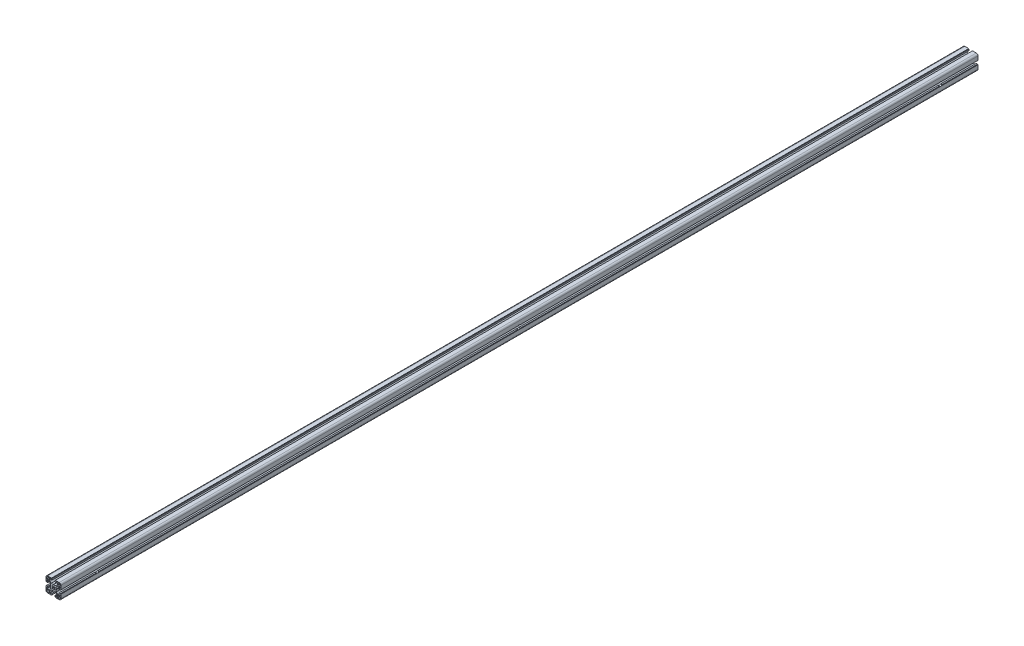
SolidWorks part; units mm, degrees
material "6061 GB/T6892-2006"
ref_plane "前视" through (0, 0, 0) normal (0, 0, 1) x (1, 0, 0)
ref_plane "上视" through (0, 0, 0) normal (0, 1, 0) x (1, 0, 0)
ref_plane "右视" through (0, 0, 0) normal (1, 0, 0) x (0, 0, -1)
sketch "草图1" plane through (0, 0, 0) normal (0, 0, 1) x (1, 0, 0)
  line L0 (-18.9995, -4.1003) -> (-18.9995, -5.1003)
  line L1 (-18.9995, -5.1003) -> (-19.9995, -5.1003)
  line L2 (-19.9995, -5.1003) -> (-19.9995, -15.5003)
  line L3 (-15.4995, -20.0003) -> (-5.0995, -20.0003)
  line L4 (-5.0995, -20.0003) -> (-5.0995, -19.0003)
  line L5 (-5.0995, -19.0003) -> (-4.0995, -19.0003)
  line L6 (-4.0995, -19.0003) -> (-4.0995, -15.5003)
  line L7 (-4.0995, -15.5003) -> (-6.5995, -15.5003)
  line L8 (-6.5995, -15.5003) -> (-6.5995, -16.5003)
  line L9 (-7.5995, -17.5003) -> (-9.7995, -17.5003)
  line L10 (-10.2995, -17.0003) -> (-10.2995, -11.9973)
  line L11 (-10.2995, -11.9973) -> (-5.9025, -7.6003)
  line L12 (-5.9025, -7.6003) -> (-0.5195, -7.6003)
  line L13 (-0.5195, -7.6003) -> (0.0005, -7.3003)
  line L14 (0.0005, -7.3003) -> (0.5195, -7.6003)
  line L15 (0.5195, -7.6003) -> (5.9035, -7.6003)
  line L16 (5.9035, -7.6003) -> (10.3005, -11.9973)
  line L17 (10.3005, -11.9973) -> (10.3005, -17.0003)
  line L18 (9.8005, -17.5003) -> (7.6005, -17.5003)
  line L19 (6.6005, -16.5003) -> (6.6005, -15.5003)
  line L20 (6.6005, -15.5003) -> (4.1005, -15.5003)
  line L21 (4.1005, -15.5003) -> (4.1005, -19.0003)
  line L22 (4.1005, -19.0003) -> (5.1005, -19.0003)
  line L23 (5.1005, -19.0003) -> (5.1005, -20.0003)
  line L24 (5.1005, -20.0003) -> (15.5005, -20.0003)
  line L25 (20.0005, -15.5003) -> (20.0005, -5.1003)
  line L26 (20.0005, -5.1003) -> (19.0005, -5.1003)
  line L27 (19.0005, -5.1003) -> (19.0005, -4.1003)
  line L28 (19.0005, -4.1003) -> (15.5005, -4.1003)
  line L29 (15.5005, -4.1003) -> (15.5005, -6.6003)
  line L30 (15.5005, -6.6003) -> (16.5005, -6.6003)
  line L31 (17.5005, -7.6003) -> (17.5005, -9.8003)
  line L32 (17.0005, -10.3003) -> (11.9975, -10.3003)
  line L33 (11.9975, -10.3003) -> (7.6005, -5.9033)
  line L34 (7.6005, -5.9033) -> (7.6005, -0.5203)
  line L35 (7.6005, -0.5203) -> (7.3005, -0.0003)
  line L36 (7.3005, -0.0003) -> (7.6005, 0.5197)
  line L37 (7.6005, 0.5197) -> (7.6005, 5.9027)
  line L38 (7.6005, 5.9027) -> (11.9975, 10.2997)
  line L39 (11.9975, 10.2997) -> (17.0005, 10.2997)
  line L40 (17.5005, 9.7997) -> (17.5005, 7.5997)
  line L41 (16.5005, 6.5997) -> (15.5005, 6.5997)
  line L42 (15.5005, 6.5997) -> (15.5005, 4.0997)
  line L43 (15.5005, 4.0997) -> (19.0005, 4.0997)
  line L44 (19.0005, 4.0997) -> (19.0005, 5.0997)
  line L45 (19.0005, 5.0997) -> (20.0005, 5.0997)
  line L46 (20.0005, 5.0997) -> (20.0005, 15.4997)
  line L47 (15.5005, 19.9997) -> (5.1005, 19.9997)
  line L48 (5.1005, 19.9997) -> (5.1005, 18.9997)
  line L49 (5.1005, 18.9997) -> (4.1005, 18.9997)
  line L50 (4.1005, 18.9997) -> (4.1005, 15.4997)
  line L51 (4.1005, 15.4997) -> (6.6005, 15.4997)
  line L52 (7.6005, 17.4997) -> (9.8005, 17.4997)
  line L53 (10.3005, 16.9997) -> (10.3005, 11.9967)
  line L54 (10.3005, 11.9967) -> (5.9035, 7.5997)
  line L55 (5.9035, 7.5997) -> (0.5195, 7.5997)
  line L56 (0.5195, 7.5997) -> (0.0005, 7.2997)
  line L57 (0.0005, 7.2997) -> (-0.5195, 7.5997)
  line L58 (-0.5195, 7.5997) -> (-5.9025, 7.5997)
  line L59 (-5.9025, 7.5997) -> (-10.2995, 11.9967)
  line L60 (-10.2995, 11.9967) -> (-10.2995, 16.9997)
  line L61 (-9.7995, 17.4997) -> (-7.5995, 17.4997)
  line L62 (-6.5995, 16.4997) -> (-6.5995, 15.4997)
  line L63 (-6.5995, 15.4997) -> (-4.0995, 15.4997)
  line L64 (-4.0995, 15.4997) -> (-4.0995, 18.9997)
  line L65 (-4.0995, 18.9997) -> (-5.0995, 18.9997)
  line L66 (-5.0995, 18.9997) -> (-5.0995, 19.9997)
  line L67 (-5.0995, 19.9997) -> (-15.4995, 19.9997)
  line L68 (-19.9995, 15.4997) -> (-19.9995, 5.0997)
  line L69 (-19.9995, 5.0997) -> (-18.9995, 5.0997)
  line L70 (-18.9995, 5.0997) -> (-18.9995, 4.0997)
  line L71 (-18.9995, 4.0997) -> (-15.4995, 4.0997)
  line L72 (-15.4995, 4.0997) -> (-15.4995, 6.5997)
  line L73 (-15.4995, 6.5997) -> (-16.4995, 6.5997)
  line L74 (-17.4995, 7.5997) -> (-17.4995, 9.7997)
  line L75 (-16.9995, 10.2997) -> (-11.9965, 10.2997)
  line L76 (-11.9965, 10.2997) -> (-7.5995, 5.9027)
  line L77 (-7.5995, 5.9027) -> (-7.5995, 0.5197)
  line L78 (-7.5995, 0.5197) -> (-7.2995, -0.0003)
  line L79 (-7.2995, -0.0003) -> (-7.5995, -0.5203)
  line L80 (-7.5995, -0.5203) -> (-7.5995, -5.9033)
  line L81 (-7.5995, -5.9033) -> (-11.9965, -10.3003)
  line L82 (-11.9965, -10.3003) -> (-16.9995, -10.3003)
  line L83 (-17.4995, -9.8003) -> (-17.4995, -7.6003)
  line L84 (-16.4995, -6.6003) -> (-15.4995, -6.6003)
  line L85 (-15.4995, -6.6003) -> (-15.4995, -4.1003)
  line L86 (-15.4995, -4.1003) -> (-18.9995, -4.1003)
  line L87 (15.5005, -18.0003) -> (11.8005, -18.0003)
  line L88 (11.8005, -18.0003) -> (11.8005, -11.8003)
  line L89 (11.8005, -11.8003) -> (18.0005, -11.8003)
  line L90 (18.0005, -11.8003) -> (18.0005, -15.5003)
  line L91 (18.0005, 11.7997) -> (11.8005, 11.7997)
  line L92 (11.8005, 11.7997) -> (11.8005, 17.9997)
  line L93 (11.8005, 17.9997) -> (15.5005, 17.9997)
  line L94 (18.0005, 15.4997) -> (18.0005, 11.7997)
  line L95 (-1.8145, -2.8753) -> (-3.0044, -4.0665)
  line L96 (-3.0044, -4.0665) -> (-4.0656, -3.0052)
  line L97 (-4.0656, -3.0052) -> (-2.8745, -1.8153)
  line L98 (-2.8745, 1.8147) -> (-4.0644, 3.0058)
  line L99 (-4.0644, 3.0058) -> (-3.0044, 4.0658)
  line L100 (-3.0044, 4.0658) -> (-1.8145, 2.8747)
  line L101 (1.8145, 2.8747) -> (3.0055, 4.0657)
  line L102 (3.0055, 4.0657) -> (4.0666, 3.0045)
  line L103 (4.0666, 3.0045) -> (2.8755, 1.8147)
  line L104 (2.8755, -1.8153) -> (4.0666, -3.0052)
  line L105 (4.0666, -3.0052) -> (3.0055, -4.0663)
  line L106 (3.0055, -4.0663) -> (1.8145, -2.8753)
  line L107 (-17.9995, -15.5003) -> (-17.9995, -11.8003)
  line L108 (-17.9995, -11.8003) -> (-11.7995, -11.8003)
  line L109 (-11.7995, -11.8003) -> (-11.7995, -18.0003)
  line L110 (-11.7995, -18.0003) -> (-15.4995, -18.0003)
  line L111 (-11.7995, 17.9997) -> (-11.7995, 11.7997)
  line L112 (-11.7995, 11.7997) -> (-17.9995, 11.7997)
  line L113 (-17.9995, 11.7997) -> (-17.9995, 15.4997)
  line L114 (-15.4995, 17.9997) -> (-11.7995, 17.9997)
  arc A0 (-19.9995, -15.5003) -> (-15.4995, -20.0003) centre (-15.4995, -15.5003) ccw
  arc A1 (-6.5995, -16.5003) -> (-7.5995, -17.5003) centre (-7.5995, -16.5003) cw
  arc A2 (-9.7995, -17.5003) -> (-10.2995, -17.0003) centre (-9.7995, -17.0003) cw
  arc A3 (10.3005, -17.0003) -> (9.8005, -17.5003) centre (9.8005, -17.0003) cw
  arc A4 (7.6005, -17.5003) -> (6.6005, -16.5003) centre (7.6005, -16.5003) cw
  arc A5 (15.5005, -20.0003) -> (20.0005, -15.5003) centre (15.5005, -15.5003) ccw
  arc A6 (16.5005, -6.6003) -> (17.5005, -7.6003) centre (16.5005, -7.6003) cw
  arc A7 (17.5005, -9.8003) -> (17.0005, -10.3003) centre (17.0005, -9.8003) cw
  arc A8 (17.0005, 10.2997) -> (17.5005, 9.7997) centre (17.0005, 9.7997) cw
  arc A9 (17.5005, 7.5997) -> (16.5005, 6.5997) centre (16.5005, 7.5997) cw
  arc A10 (20.0005, 15.4997) -> (15.5005, 19.9997) centre (15.5005, 15.4997) ccw
  arc A11 (6.6005, 15.4997) -> (6.6005, 16.4997) centre (7.1003, 15.9997) cw
  arc A12 (6.6005, 16.4997) -> (7.6005, 17.4997) centre (7.6005, 16.4997) cw
  arc A13 (9.8005, 17.4997) -> (10.3005, 16.9997) centre (9.8005, 16.9997) cw
  arc A14 (-10.2995, 16.9997) -> (-9.7995, 17.4997) centre (-9.7995, 16.9997) cw
  arc A15 (-7.5995, 17.4997) -> (-6.5995, 16.4997) centre (-7.5995, 16.4997) cw
  arc A16 (-15.4995, 19.9997) -> (-19.9995, 15.4997) centre (-15.4995, 15.4997) ccw
  arc A17 (-16.4995, 6.5997) -> (-17.4995, 7.5997) centre (-16.4995, 7.5997) cw
  arc A18 (-17.4995, 9.7997) -> (-16.9995, 10.2997) centre (-16.9995, 9.7997) cw
  arc A19 (-16.9995, -10.3003) -> (-17.4995, -9.8003) centre (-16.9995, -9.8003) cw
  arc A20 (-17.4995, -7.6003) -> (-16.4995, -6.6003) centre (-16.4995, -7.6003) cw
  arc A21 (18.0005, -15.5003) -> (15.5005, -18.0003) centre (15.5005, -15.5003) cw
  arc A22 (15.5005, 17.9997) -> (18.0005, 15.4997) centre (15.5005, 15.4997) cw
  arc A23 (-2.8745, -1.8153) -> (-2.8745, 1.8147) centre (0.0005, -0.0003) cw
  arc A24 (-1.8145, 2.8747) -> (1.8145, 2.8747) centre (0, -0.0007) cw
  arc A25 (2.8755, 1.8147) -> (2.8755, -1.8153) centre (0.0005, -0.0003) cw
  arc A26 (1.8145, -2.8753) -> (-1.8145, -2.8753) centre (0, 0) cw
  arc A27 (-15.4995, -18.0003) -> (-17.9995, -15.5003) centre (-15.4995, -15.5003) cw
  arc A28 (-17.9995, 15.4997) -> (-15.4995, 17.9997) centre (-15.4995, 15.4997) cw
extrude "凸台-拉伸1" add sketch "草图1" against normal blind 2470
hole_wizard "打孔尺寸(%根据)内六角圆柱头螺钉的类型2" positions "草图2" profile "草图3" counterbore size "M6" standard "GB" end condition through all
sketch "草图2" plane through (20.0005, 0, 0) normal (1, 0, 0) x (0, 0, -1)
  line L0 (2470, -0.0003) -> (0, -0.0003) construction
  line L1 (2470, 0.5197) -> (0, 0.5197) construction
  point P0 (2370, -0.0003)
  point P4 (1235, 0.5197)
  point P8 (100, -0.0003)
  dimension "D1" = 100
  dimension "D2" = 100
sketch "草图3" plane through (20.0005, -0.0003, -2370) normal (0, 1, 0) x (0, 0, -1)
  line L0 (0, 0) -> (0, 40)
  line L1 (0, 40) -> (3.3, 40)
  line L3 (3.3, 40) -> (3.3, 6.8)
  line L4 (3.3, 6.8) -> (5.5, 6.8)
  line L5 (5.5, 6.8) -> (5.5, 0)
  line L7 (5.5, 0) -> (0, 0)
  line L11 (0, -6.35) -> (0, 107.95) construction
  dimension "通孔孔直径" = 6.6
  dimension "通孔孔深度" = 40
  dimension "柱形沉头孔直径" = 11
  dimension "柱形沉头孔深度" = 6.8
hole_wizard "打孔尺寸(%根据)内六角圆柱头螺钉的类型2" positions "草图4" profile "草图5" counterbore size "M6" standard "GB" end condition through all
sketch "草图4" plane through (-19.9995, 0, 0) normal (-1, 0, 0) x (0, 0, 1)
  point P0 (-100, -0.0003)
  point P3 (-1235, 0.5197)
  point P6 (-2370, -0.0003)
sketch "草图5" plane through (-19.9995, -0.0003, -100) normal (0, 1, 0) x (0, 0, 1)
  line L0 (0, 0) -> (0, 40)
  line L1 (0, 40) -> (3.3, 40)
  line L3 (3.3, 40) -> (3.3, 6.8)
  line L4 (3.3, 6.8) -> (5.5, 6.8)
  line L5 (5.5, 6.8) -> (5.5, 0)
  line L7 (5.5, 0) -> (0, 0)
  line L11 (0, -6.35) -> (0, 107.95) construction
  dimension "通孔孔直径" = 6.6
  dimension "通孔孔深度" = 40
  dimension "柱形沉头孔直径" = 11
  dimension "柱形沉头孔深度" = 6.8
